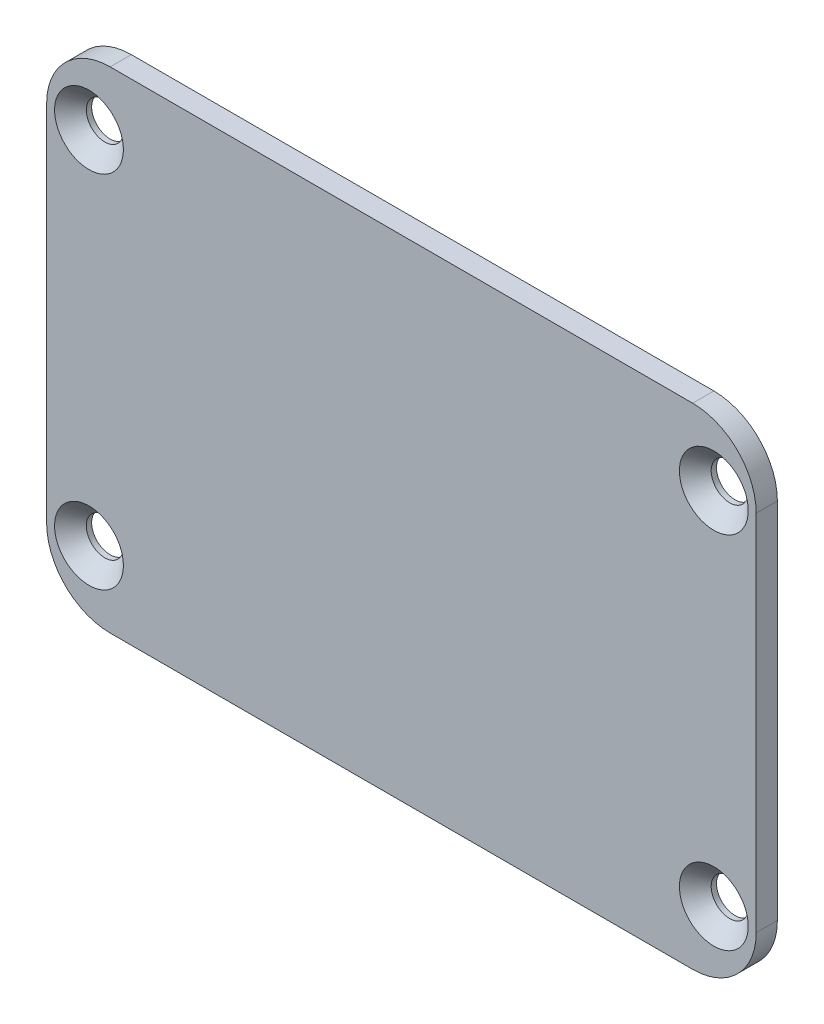
SolidWorks part; units mm, degrees
material "6061 合金"
ref_plane "前视基准面" through (0, 0, 0) normal (0, 0, 1) x (1, 0, 0)
ref_plane "上视基准面" through (0, 0, 0) normal (0, 1, 0) x (1, 0, 0)
ref_plane "右视基准面" through (0, 0, 0) normal (1, 0, 0) x (0, 0, -1)
sketch "草图1" plane through (0, 0, 0) normal (0, 0, 1) x (1, 0, 0)
  line L1 (-33.5, 23.15) -> (33.5, 23.15)
  line L2 (-33.5, 23.15) -> (-33.5, -23.15)
  line L3 (-33.5, -23.15) -> (33.5, -23.15)
  line L4 (33.5, 23.15) -> (33.5, -23.15)
  dimension "D1" = 67
  dimension "D2" = 46.3
extrude "拉伸1" add sketch "草图1" along normal blind 2
fillet "圆角1" radius 6 4 edges at (-33.5, -23.15, 1) (33.5, -23.15, 1) (33.5, 23.15, 1) (-33.5, 23.15, 1)
hole_wizard "孔1" positions "3D草图1" profile "草图2" legacy
sketch3d "3D草图1"
  point P0 (-29.5, -17, 2)
sketch "草图2" plane through (-29.5, -17, 2) normal (1, 0, 0) x (0, -1, 0)
  line L0 (0, 0) -> (0, 10)
  line L1 (0, 10) -> (1.75, 10)
  line L2 (1.75, 10) -> (1.75, 1.5)
  line L3 (1.75, 1.5) -> (3.25, 0)
  line L4 (3.25, 0) -> (0, 0)
  line L5 (0, -6.4453) -> (0, 115.525) construction
  line L6 (-1.75, 1.5) -> (-3.25, 0) construction
  dimension "眻噤" = 3.5
  dimension "旮僅" = 10
  dimension "袪諧褒僅" = 90
  dimension "袪諧眻噤" = 6.5
pattern_linear "阵列(线性)1" count 2 spacing 34 along (0, 1, 0) count 2 spacing 59 along (1, 0, 0) of "孔1"
